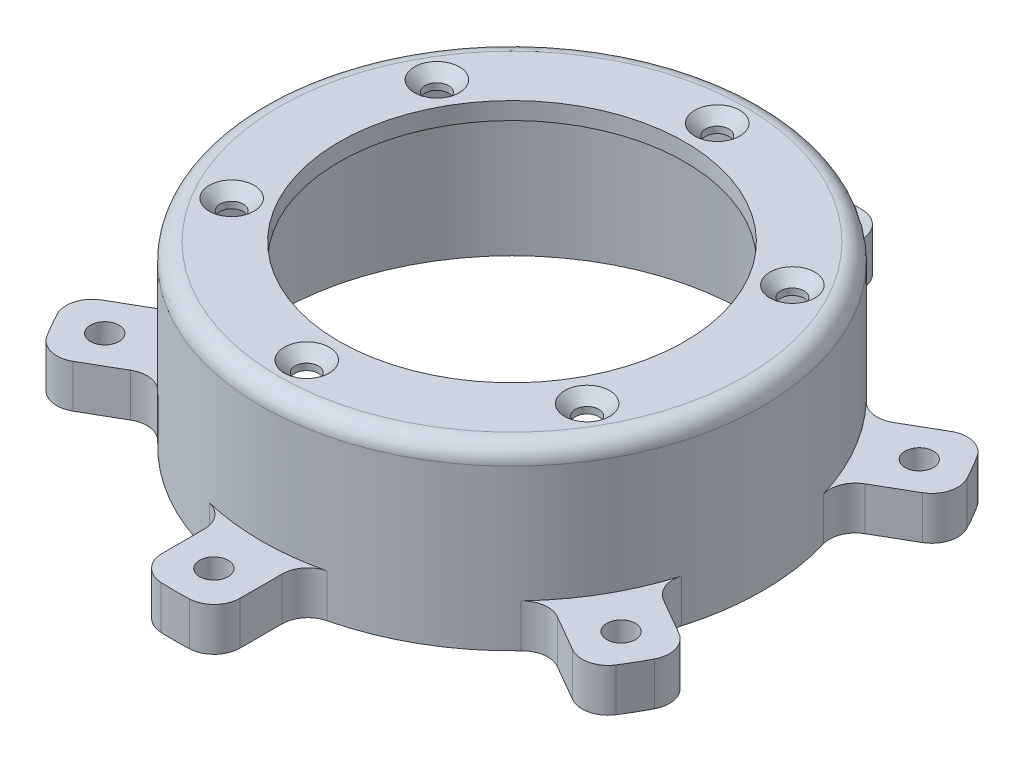
SolidWorks part; units mm, degrees
material "6061 合金"
ref_plane "前视基准面" through (0, 0, 0) normal (0, 0, 1) x (1, 0, 0)
ref_plane "上视基准面" through (0, 0, 0) normal (0, 1, 0) x (1, 0, 0)
ref_plane "右视基准面" through (0, 0, 0) normal (1, 0, 0) x (0, 0, -1)
sketch "草图1" plane through (0, 0, 0) normal (0, 1, 0) x (1, 0, 0)
  circle A0 centre (0, 0) radius 23.75 construction
  circle A1 centre (0, 0) radius 20
  circle A2 centre (0, 0) radius 29
  circle A3 centre (0, 23.75) radius 1.3
  circle A4 centre (20.5681, 11.875) radius 1.3
  circle A5 centre (20.5681, -11.875) radius 1.3
  circle A6 centre (0, -23.75) radius 1.3
  circle A7 centre (-20.5681, -11.875) radius 1.3
  circle A8 centre (-20.5681, 11.875) radius 1.3
  point P19 (0, 0)
  dimension "D1" = 58
  dimension "D2" = 47.5
  dimension "D3" = 40
  dimension "D4" = 2.6
  dimension "D5" = 6
extrude "凸台-拉伸1" add sketch "草图1" against normal blind 2
sketch "草图2" plane through (0, -2, 0) normal (0, -1, 0) x (1, 0, 0)
  circle A0 centre (0, 0) radius 29 construction
  circle A1 centre (0, 0) radius 29
  circle A2 centre (0, 0) radius 27
  dimension "D1" = 2
extrude "凸台-拉伸2" add sketch "草图2" along normal blind 18.5
sketch "草图3" plane through (0, -20.5, 0) normal (0, -1, 0) x (1, 0, 0)
  line L0 (-4.5, 35.9687) -> (-4.5, 28.6487)
  line L1 (4.5, 35.9687) -> (4.5, 28.6487)
  line L2 (28.8998, 21.8815) -> (22.5605, 18.2215)
  line L3 (33.3998, 14.0873) -> (27.0605, 10.4273)
  line L4 (33.3998, -14.0873) -> (27.0605, -10.4273)
  line L5 (28.8998, -21.8815) -> (22.5605, -18.2215)
  line L6 (4.5, -35.9687) -> (4.5, -28.6487)
  line L7 (-4.5, -35.9687) -> (-4.5, -28.6487)
  line L8 (-28.8998, -21.8815) -> (-22.5605, -18.2215)
  line L9 (-33.3998, -14.0873) -> (-27.0605, -10.4273)
  line L10 (-33.3998, 14.0873) -> (-27.0605, 10.4273)
  line L11 (-28.8998, 21.8815) -> (-22.5605, 18.2215)
  circle A0 centre (0, 0) radius 29 construction
  arc A1 (4.5, 28.6487) -> (-4.5, 28.6487) centre (0, 0) ccw
  circle A2 centre (0, 0) radius 34.5 construction
  circle A4 centre (0, 34.5) radius 4 construction
  circle A5 centre (29.8779, 17.25) radius 4 construction
  circle A6 centre (29.8779, -17.25) radius 4 construction
  circle A7 centre (0, -34.5) radius 4 construction
  circle A8 centre (-29.8779, -17.25) radius 4 construction
  circle A9 centre (-29.8779, 17.25) radius 4 construction
  arc A10 (1.625, 38.9661) -> (-1.625, 38.9661) centre (0, 0) ccw
  arc A11 (4.5, 35.9687) -> (1.625, 38.9661) centre (1.5, 35.9687) ccw
  arc A12 (-4.5, 35.9687) -> (-1.625, 38.9661) centre (-1.5, 35.9687) cw
  arc A13 (27.0605, 10.4273) -> (22.5605, 18.2215) centre (0, 0) ccw
  arc A14 (28.8998, 21.8815) -> (32.9332, 20.8904) centre (30.3998, 19.2834) cw
  arc A15 (34.5582, 18.0758) -> (32.9332, 20.8904) centre (0, 0) ccw
  arc A16 (33.3998, 14.0873) -> (34.5582, 18.0758) centre (31.8998, 16.6853) ccw
  arc A17 (22.5605, -18.2215) -> (27.0605, -10.4273) centre (0, 0) ccw
  arc A18 (33.3998, -14.0873) -> (34.5582, -18.0758) centre (31.8998, -16.6853) cw
  arc A19 (32.9332, -20.8904) -> (34.5582, -18.0758) centre (0, 0) ccw
  arc A20 (28.8998, -21.8815) -> (32.9332, -20.8904) centre (30.3998, -19.2834) ccw
  arc A21 (-4.5, -28.6487) -> (4.5, -28.6487) centre (0, 0) ccw
  arc A22 (4.5, -35.9687) -> (1.625, -38.9661) centre (1.5, -35.9687) cw
  arc A23 (-1.625, -38.9661) -> (1.625, -38.9661) centre (0, 0) ccw
  arc A24 (-4.5, -35.9687) -> (-1.625, -38.9661) centre (-1.5, -35.9687) ccw
  arc A25 (-27.0605, -10.4273) -> (-22.5605, -18.2215) centre (0, 0) ccw
  arc A26 (-28.8998, -21.8815) -> (-32.9332, -20.8904) centre (-30.3998, -19.2834) cw
  arc A27 (-34.5582, -18.0758) -> (-32.9332, -20.8904) centre (0, 0) ccw
  arc A28 (-33.3998, -14.0873) -> (-34.5582, -18.0758) centre (-31.8998, -16.6853) ccw
  arc A29 (-22.5605, 18.2215) -> (-27.0605, 10.4273) centre (0, 0) ccw
  arc A30 (-33.3998, 14.0873) -> (-34.5582, 18.0758) centre (-31.8998, 16.6853) cw
  arc A31 (-32.9332, 20.8904) -> (-34.5582, 18.0758) centre (0, 0) ccw
  arc A32 (-28.8998, 21.8815) -> (-32.9332, 20.8904) centre (-30.3998, 19.2834) ccw
  circle A33 centre (0, 0) radius 29.5 construction
  circle A34 centre (0, 34.5) radius 2 construction
  point P18 (0, 0)
  point P68 (0, 0)
  dimension "D1" = 8
  dimension "D3" = 5
  dimension "D4" = 78
  dimension "D6" = 3
  dimension "D8" = 0.5
  dimension "D5" = 4
  dimension "5.5" = 4.5
  dimension "D2" = 6
  dimension "D7" = 6
extrude "凸台-拉伸3" add sketch "草图3" against normal blind 5
sketch "草图4" plane through (0, -20.5, 0) normal (0, -1, 0) x (1, 0, 0)
  point P0 (-29.8779, 17.25)
  point P2 (-29.8779, -17.25)
  point P4 (0, -34.5)
  point P6 (29.8779, -17.25)
  point P8 (29.8779, 17.25)
  point P10 (0, 34.5)
hole_wizard "M4 螺纹孔1" positions "草图4" profile "草图5" tap size "M4" standard "GB" end condition through all
sketch "草图5" plane through (-29.8779, -20.5, 17.25) normal (1, 0, 0) x (0, 0, -1)
  line L0 (0, 0) -> (0, 20.5)
  line L1 (0, 20.5) -> (1.65, 20.5)
  line L2 (1.65, 20.5) -> (1.65, 0)
  line L5 (1.65, 0) -> (0, 0)
  line L11 (0, -6.35) -> (0, 107.95) construction
  dimension "通孔螺纹孔钻头直径" = 3.3
  dimension "通孔螺纹孔钻头深度" = 20.5
cosmetic thread "孔螺纹线1"
cosmetic thread "孔螺纹线2"
cosmetic thread "孔螺纹线3"
cosmetic thread "孔螺纹线4"
cosmetic thread "孔螺纹线5"
cosmetic thread "孔螺纹线6"
fillet "圆角1" radius 3 12 edges at (-22.5605, -18, 18.2215) (-27.0605, -18, 10.4273) (-27.0605, -18, -10.4273) (-22.5605, -18, -18.2215) (-4.5, -18, -28.6487) (4.5, -18, -28.6487) (22.5605, -18, -18.2215) (27.0605, -18, -10.4273) (27.0605, -18, 10.4273) (22.5605, -18, 18.2215) (4.5, -18, 28.6487) (-4.5, -18, 28.6487)
fillet "圆角2" radius 2 1 edges at (0, 0, 29)
hole_wizard "M3 内六角花形沉头螺钉的锥形沉头孔1" positions "草图9" profile "草图7" countersink size "M6" standard "GB" end condition through all
sketch "草图9" plane through (0, 0, 0) normal (0, 1, 0) x (1, 0, 0)
  point P0 (0, 23.75)
  point P3 (20.5681, 11.875)
  point P6 (20.5681, -11.875)
  point P9 (0, -23.75)
  point P12 (-20.5681, -11.875)
  point P15 (-20.5681, 11.875)
sketch "草图7" plane through (0, 0, -23.75) normal (1, 0, 0) x (0, 0, 1)
  line L0 (0, 0) -> (0, 20.5)
  line L1 (0, 20.5) -> (1.35, 20.5)
  line L2 (1.35, 20.5) -> (1.35, 1.25)
  line L3 (1.35, 1.25) -> (2.6, 0)
  line L5 (2.6, 0) -> (0, 0)
  line L6 (-1.35, 1.25) -> (-2.6, 0) construction
  line L11 (0, -6.35) -> (0, 107.95) construction
  dimension "通孔孔直径" = 2.7
  dimension "通孔孔深度" = 20.5
  dimension "近端锥形沉头孔直径" = 5.2
  dimension "近端锥形沉头孔角度" = 90
